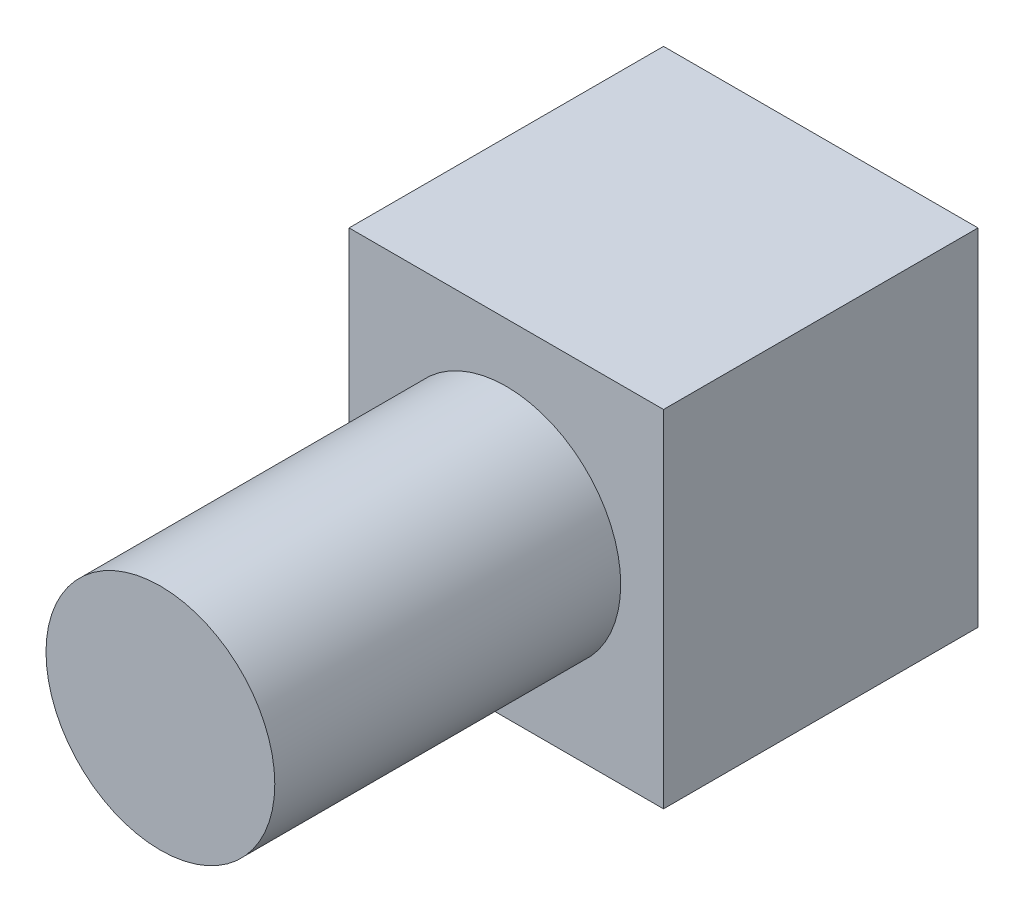
from build123d import *

# Parameters (mm, degrees)
SKETCH1_W           = 50
SKETCH1_H           = 50
BOSS_EXTRUDE1_DEPTH = 55
SKETCH2_R           = 18.189043711
BOSS_EXTRUDE2_DEPTH = 55


with BuildPart() as part:
    # Sketch1 → Boss-Extrude1 (new body)
    with BuildSketch(Plane(origin=(0, 0, 0), x_dir=(1, 0, 0), z_dir=(0, 1, 0))):
        Rectangle(SKETCH1_W, SKETCH1_H)
    extrude(amount=BOSS_EXTRUDE1_DEPTH)

    # Sketch2 → Boss-Extrude2 (add)
    with BuildSketch(Plane.XY.offset(25)):
        with Locations((0, 27.5)):
            Circle(SKETCH2_R)
    extrude(amount=BOSS_EXTRUDE2_DEPTH)


solid = part.part
